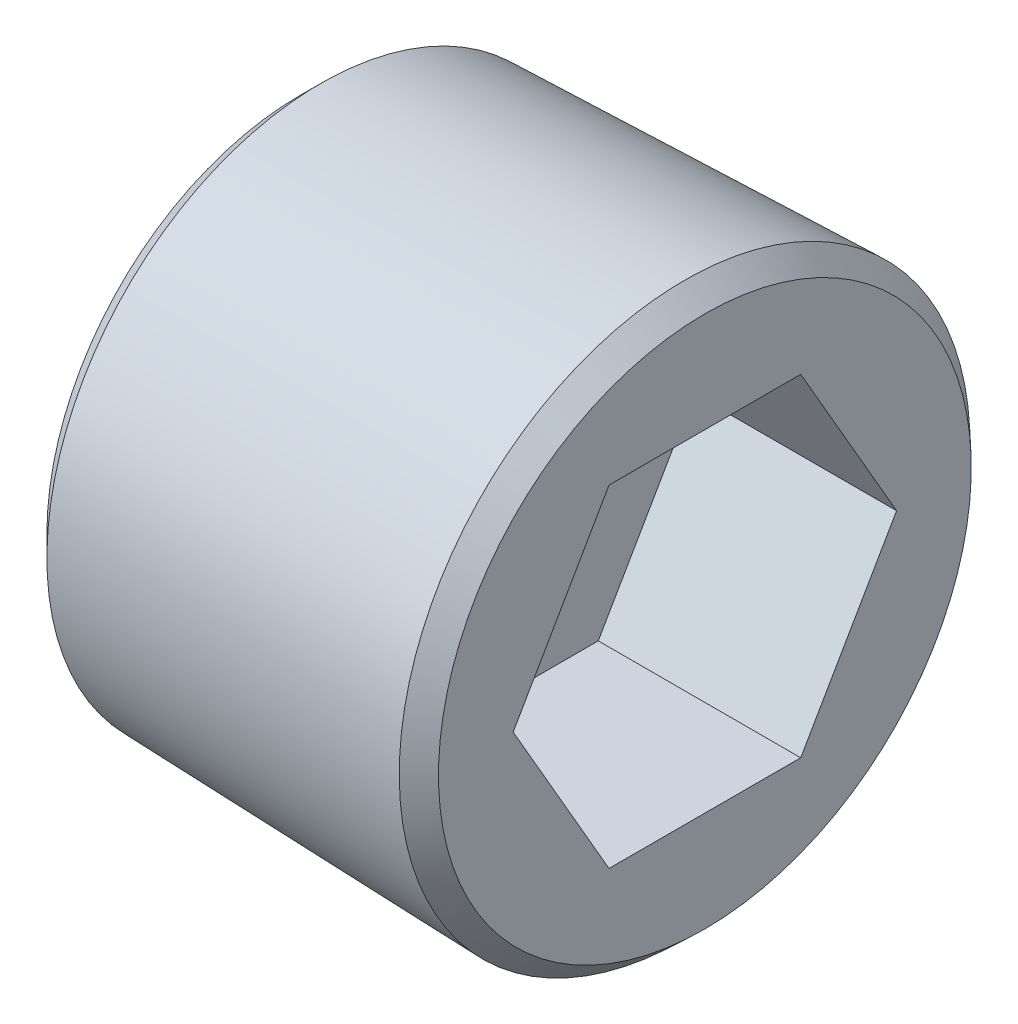
SolidWorks part; units mm, degrees
material "黄铜"
ref_plane "前视基准面" through (0, 0, 0) normal (0, 0, 1) x (1, 0, 0)
ref_plane "上视基准面" through (0, 0, 0) normal (0, 1, 0) x (1, 0, 0)
ref_plane "右视基准面" through (0, 0, 0) normal (1, 0, 0) x (0, 0, -1)
sketch "草图1" plane through (0, 0, 0) normal (0, 0, 1) x (1, 0, 0)
  line L0 (0, 0) -> (-10, 0) construction
  line L1 (0, 0) -> (0, 6.75)
  line L2 (0, 6.75) -> (10, 7.0643)
  line L3 (10, 7.0643) -> (10, 0)
  line L4 (10, 0) -> (0, 0)
  dimension "D1" = 1.8
  dimension "D2" = 13.5
  dimension "D3" = 10
revolve "旋转1" add sketch "草图1" angle 360 about L0
sketch "草图2" plane through (10, 0, 0) normal (1, 0, 0) x (0, 0, -1)
  line L1 (2.3671, -4.1) -> (4.7343, 0)
  line L2 (4.7343, 0) -> (2.3671, 4.1)
  line L3 (2.3671, 4.1) -> (-2.3671, 4.1)
  line L4 (-2.3671, 4.1) -> (-4.7343, 0)
  line L5 (-4.7343, 0) -> (-2.3671, -4.1)
  line L6 (-2.3671, -4.1) -> (2.3671, -4.1)
  circle A0 centre (0, 0) radius 4.1 construction
  dimension "D1" = 8.2
extrude "切除-拉伸1" cut sketch "草图2" against normal blind 5
chamfer "倒角1" distance 0.5 angle 45 2 edges at (10, 7.0643, 0) (0, 6.75, 0)
